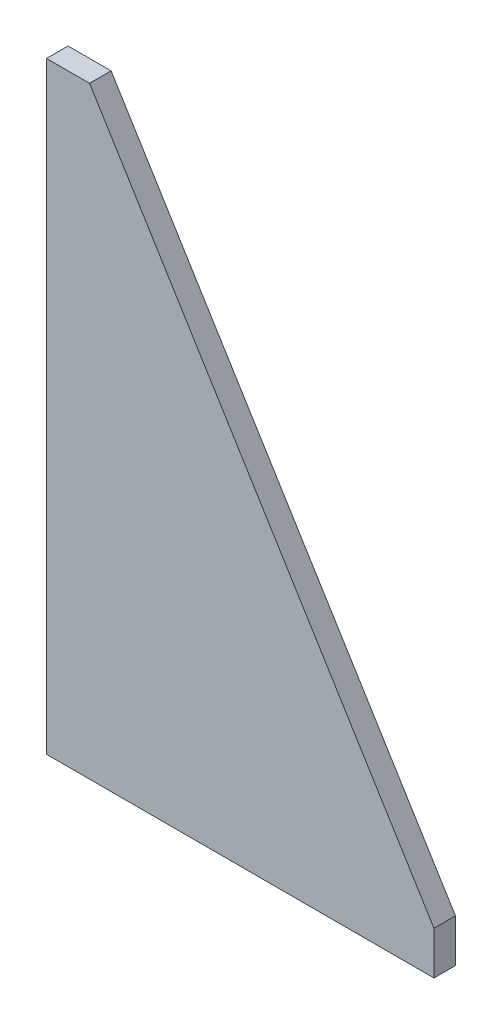
SolidWorks part; units mm, degrees
ref_plane "Front Plane" through (0, 0, 0) normal (0, 0, 1) x (1, 0, 0)
ref_plane "Top Plane" through (0, 0, 0) normal (0, 1, 0) x (1, 0, 0)
ref_plane "Right Plane" through (0, 0, 0) normal (1, 0, 0) x (0, 0, -1)
other "Configuration Table"
sketch "Sketch1" plane through (0, 0, 0) normal (0, 0, 1) x (1, 0, 0)
  line L0 (0, 0) -> (0, 280)
  line L1 (0, 280) -> (20, 280)
  line L2 (20, 280) -> (180, 20)
  line L3 (180, 20) -> (180, 0)
  line L4 (180, 0) -> (0, 0)
  dimension "D1" = 180
  dimension "D2" = 280
  dimension "D3" = 20
  dimension "D4" = 20
extrude "Boss-Extrude1" add sketch "Sketch1" along normal blind 10
